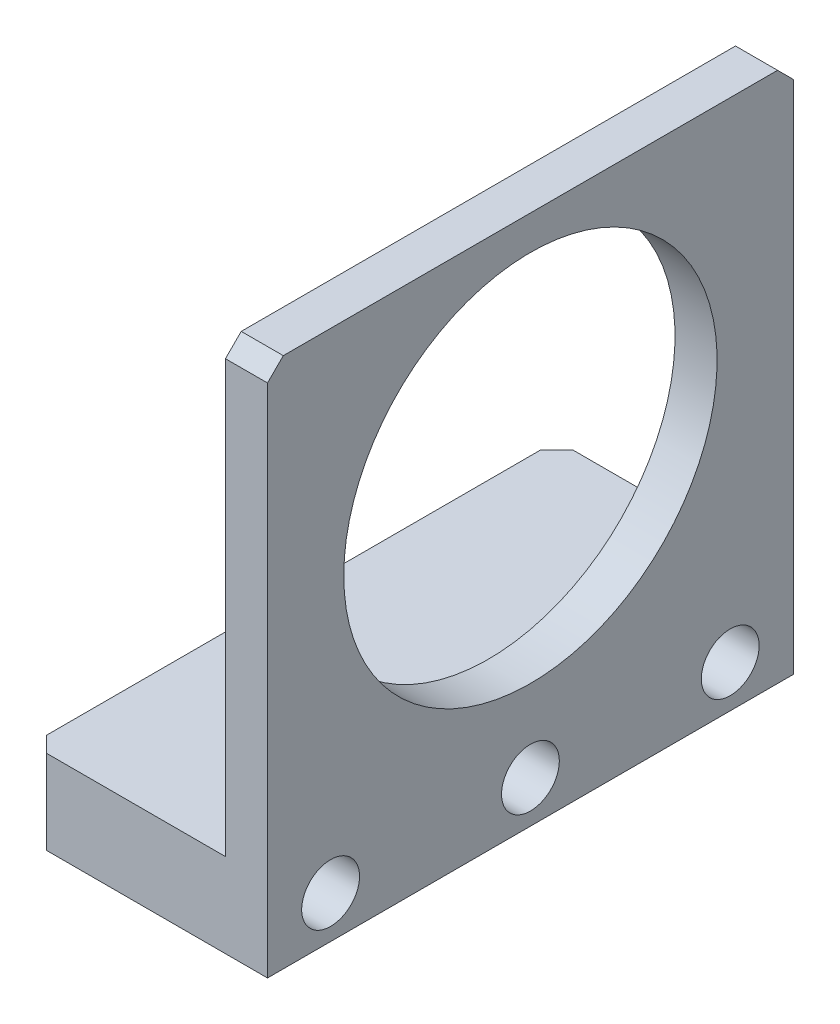
SolidWorks part; units mm, degrees
ref_plane "前视基准面" through (0, 0, 0) normal (0, 0, 1) x (1, 0, 0)
ref_plane "上视基准面" through (0, 0, 0) normal (0, 1, 0) x (1, 0, 0)
ref_plane "右视基准面" through (0, 0, 0) normal (1, 0, 0) x (0, 0, -1)
sketch "草图2" plane through (409.6376, 0.5, -34.3795) normal (0, 0, 1) x (1, 0, 0)
  line L0 (-409.6376, 100.5) -> (-409.6376, -0.5)
  line L1 (-409.6376, -0.5) -> (-454.6376, -0.5)
  line L2 (-454.6376, -0.5) -> (-454.6376, 15.5)
  line L3 (-454.6376, 15.5) -> (-417.6376, 15.5)
  line L4 (-417.6376, 15.5) -> (-417.6376, 100.5)
  line L5 (-417.6376, 100.5) -> (-409.6376, 100.5)
  dimension "D2" = 8
  dimension "D3" = 16
  dimension "D4" = 85
  dimension "D5" = 37
extrude "凸台-拉伸1" add sketch "草图2" along normal mid plane 100
chamfer "倒角1" distance 3 angle 45 4 edges at (-45, 8, -84.3795) (-45, 8, 15.6205) (-4, 101, 15.6205) (-4, 101, -84.3795)
sketch "草图3" plane through (-8, 0, 0) normal (-1, 0, 0) x (0, 0, 1)
  line L0 (-34.3795, 101) -> (-34.3795, 59) construction
  line L1 (12.6205, 101) -> (-81.3795, 101) construction
  circle A0 centre (-34.3795, 59) radius 35.5
  dimension "D1" = 71
  dimension "D2" = 42
extrude "切除-拉伸1" cut sketch "草图3" against normal up to next
hole_wizard "打孔尺寸(%根据)内六角圆柱头螺钉的类型1" positions "3D草图1" profile "草图4" counterbore size "M6" standard "GB" end condition up to next
sketch3d "3D草图1"
  line L1 (0, 0, 15.6205) -> (0, 0, -84.3795) construction
  line L2 (0, 0, 15.6205) -> (0, 98, 15.6205) construction
  line L3 (0, 0, -84.3795) -> (0, 98, -84.3795) construction
  line L4 (0, 0, -34.3795) -> (0, 8, -34.3795)
  point P0 (0, 8, 3.6205)
  point P9 (0, 8, -34.3795)
  point P11 (0, 8, -72.3795)
  dimension "D1" = 8
  dimension "D2" = 12
  dimension "D3" = 12
sketch "草图4" plane through (0, 8, 3.6205) normal (0, 1, 0) x (0, 0, -1)
  line L0 (0, 0) -> (0, 45)
  line L1 (0, 45) -> (3.3, 45)
  line L3 (3.3, 45) -> (3.3, 35)
  line L4 (3.3, 35) -> (5.5, 35)
  line L5 (5.5, 35) -> (5.5, 0)
  line L7 (5.5, 0) -> (0, 0)
  line L11 (0, -6.35) -> (0, 107.95) construction
  dimension "通孔孔直径" = 6.6
  dimension "通孔孔深度" = 45
  dimension "柱形沉头孔直径" = 11
  dimension "柱形沉头孔深度" = 35
